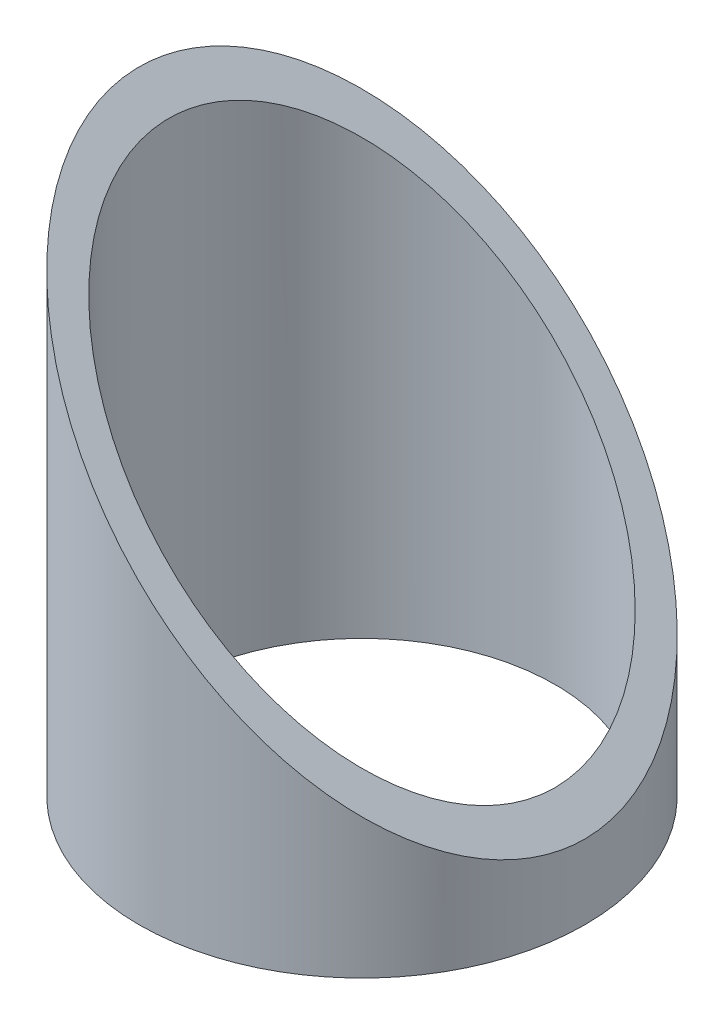
from build123d import *

# Parameters (mm, degrees)
SKETCH1_R               = 30
SKETCH1_R_2             = 26
BOSS_EXTRUDE1_DEPTH     = 70
CUT_EXTRUDE1_DEPTH      = 82.853527719
CUT_EXTRUDE1_DEPTH_BACK = 82.853527719


with BuildPart() as part:
    # Sketch1 → Boss-Extrude1 (new body)
    with BuildSketch(Plane(origin=(0, 0, 0), x_dir=(1, 0, 0), z_dir=(0, 1, 0))):
        with Locations(Location((0, 0, 0), (0, 0, 270))):
            Circle(SKETCH1_R)
        with Locations(Location((0, 0, 0), (0, 0, 270))):
            Circle(SKETCH1_R_2, mode=Mode.SUBTRACT)
    extrude(amount=BOSS_EXTRUDE1_DEPTH)

    # Sketch2 → Cut-Extrude1 (cut, two sides: drawn at the far end of the back side and taken through both)
    with BuildSketch(Plane.XY.offset(-CUT_EXTRUDE1_DEPTH_BACK)):
        Polygon((-167.455115916, 207.455115916), (-30, 70), (33.212319076, 6.787680924), (170.667434992, -130.667434992), (445.577666824, 144.24279684), (107.455115916, 482.365347748), align=None)
    extrude(amount=CUT_EXTRUDE1_DEPTH + CUT_EXTRUDE1_DEPTH_BACK, mode=Mode.SUBTRACT)


solid = part.part
